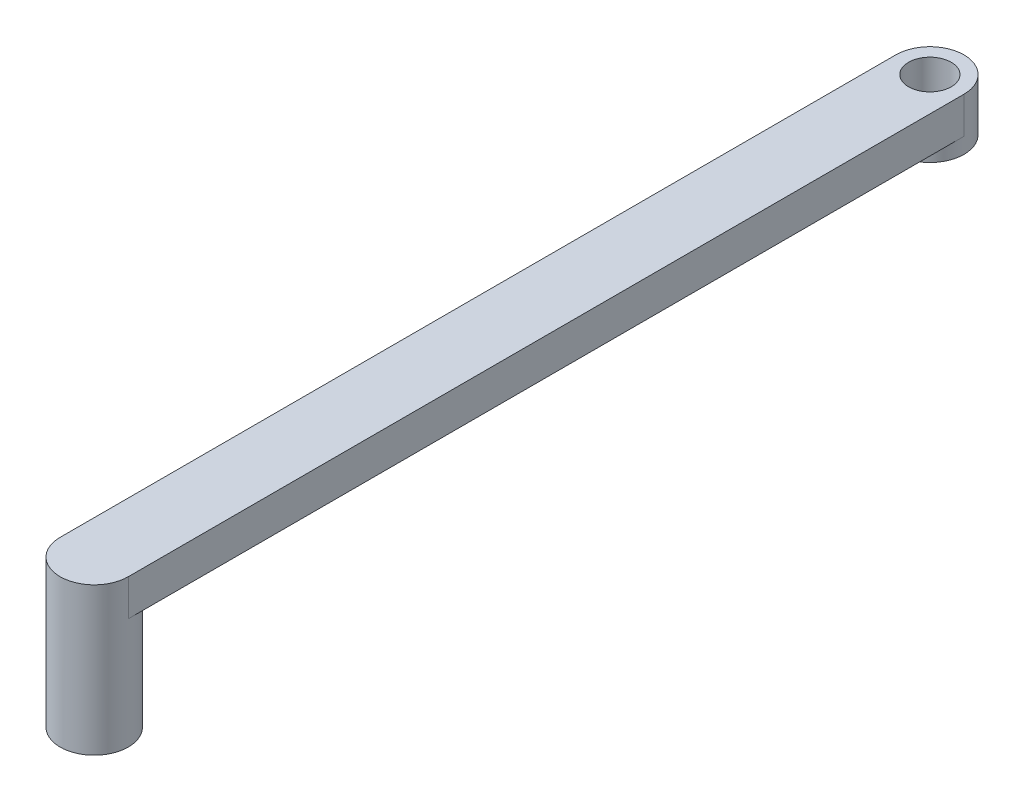
from build123d import *

# Parameters (mm, degrees)
SKETCH1_R           = 200
SKETCH1_R_2         = 125
BOSS_EXTRUDE1_DEPTH = 220
BOSS_EXTRUDE2_DEPTH = 214
SKETCH3_R           = 200
BOSS_EXTRUDE3_DEPTH = 780
SKETCH4_R           = 137.5
CUT_EXTRUDE1_DEPTH  = 604
SKETCH5_R           = 200
SKETCH5_R_2         = 90
BOSS_EXTRUDE4_DEPTH = 86
SKETCH6_R           = 200
BOSS_EXTRUDE5_DEPTH = 86


with BuildPart() as part:
    # Sketch1 → Boss-Extrude1 (new body)
    with BuildSketch(Plane(origin=(0, 0, 0), x_dir=(1, 0, 0), z_dir=(0, 1, 0))):
        with Locations(Location((0, 0, 0), (0, 0, 270))):
            Circle(SKETCH1_R)
        with Locations(Location((0, 0, 0), (0, 0, 270))):
            Circle(SKETCH1_R_2, mode=Mode.SUBTRACT)
    extrude(amount=-BOSS_EXTRUDE1_DEPTH)

    # Sketch2 → Boss-Extrude2 (add)
    with BuildSketch(Plane(origin=(0, 0, 0), x_dir=(1, 0, 0), z_dir=(0, 1, 0))):
        with BuildLine():
            ThreePointArc((200, 0), (0, -200), (-200, 0))
            Line((-200, 0), (-200, -4903.05503267))
            ThreePointArc((-200, -4903.05503267), (0, -4703.05503267), (200, -4903.05503267))
            Line((200, -4903.05503267), (200, 0))
        make_face()
    extrude(amount=-BOSS_EXTRUDE2_DEPTH)

    # Sketch3 → Boss-Extrude3 (add)
    with BuildSketch(Plane(origin=(0, 0, 0), x_dir=(1, 0, 0), z_dir=(0, 1, 0))):
        with Locations(Location((0, -4903.05503267, 0), (0, 0, 270))):
            Circle(SKETCH3_R)
    extrude(amount=-BOSS_EXTRUDE3_DEPTH)

    # Sketch4 → Cut-Extrude1 (cut)
    with BuildSketch(Plane.XZ.offset(780)):
        with Locations(Location((0, 4903.05503267, 0), (0, 0, 270))):
            Circle(SKETCH4_R)
    extrude(amount=-CUT_EXTRUDE1_DEPTH, mode=Mode.SUBTRACT)

    # Sketch5 → Boss-Extrude4 (add)
    with BuildSketch(Plane.XZ.offset(780)):
        with Locations((0, 4903.05503267)):
            Circle(SKETCH5_R)
        with Locations(Location((0, 4903.05503267, 0), (0, 0, 270))):
            Circle(SKETCH5_R_2, mode=Mode.SUBTRACT)
    extrude(amount=BOSS_EXTRUDE4_DEPTH)

    # Sketch6 → Boss-Extrude5 (add)
    with BuildSketch(Plane.XZ.offset(220)):
        Circle(SKETCH6_R)
    extrude(amount=BOSS_EXTRUDE5_DEPTH)


solid = part.part
